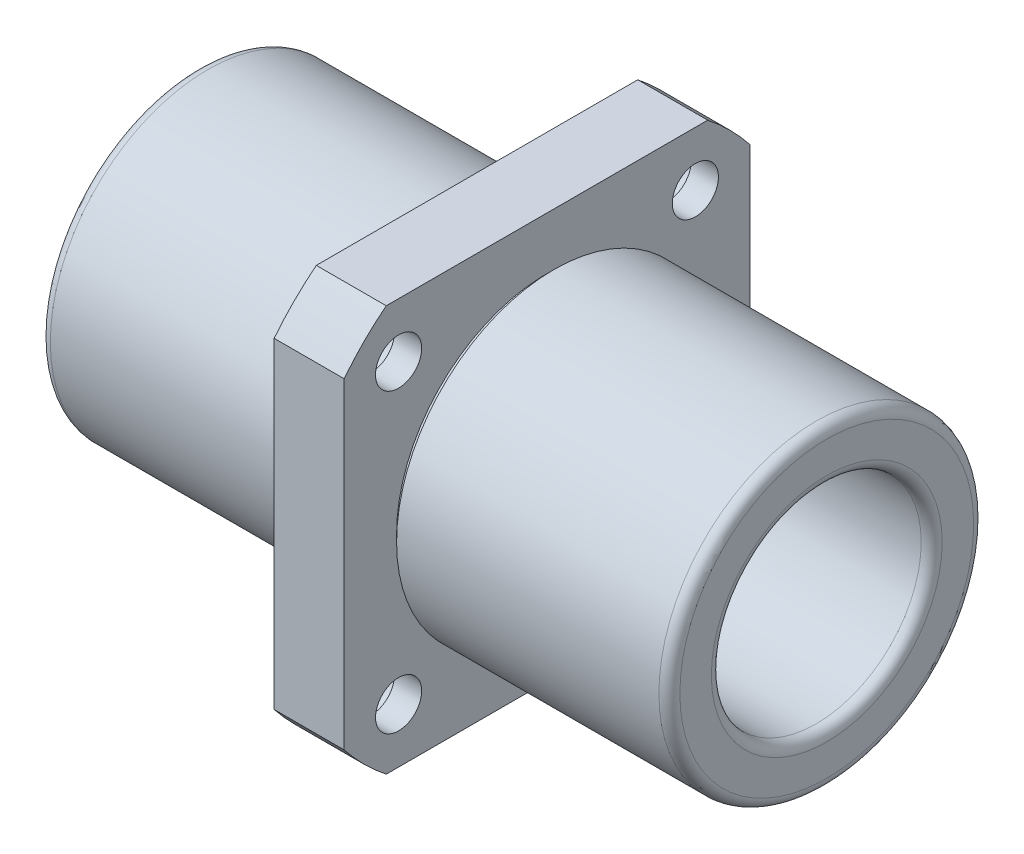
SolidWorks part; units mm, degrees
material "Q235-AF"
ref_plane "Front Plane" through (0, 0, 0) normal (0, 0, 1) x (1, 0, 0)
ref_plane "Top Plane" through (0, 0, 0) normal (0, 1, 0) x (1, 0, 0)
ref_plane "Right Plane" through (0, 0, 0) normal (1, 0, 0) x (0, 0, -1)
sketch "Sketch1" plane through (0, 0, 0) normal (0, 0, 1) x (1, 0, 0)
  line L0 (0, 37) -> (0, 21.5)
  line L1 (0, 15) -> (50, 15)
  line L2 (50, 15) -> (50, 22.5)
  line L3 (50, 22.5) -> (11, 22.5)
  line L4 (11, 22.5) -> (11, 21.5)
  line L5 (11, 21.5) -> (10, 21.5)
  line L6 (10, 21.5) -> (10, 37)
  line L7 (10, 37) -> (0, 37)
  line L8 (64, 0) -> (0, 0) construction
  line L9 (0, 21.5) -> (-1, 21.5)
  line L10 (-1, 21.5) -> (-1, 22.5)
  line L11 (-1, 22.5) -> (-40, 22.5)
  line L12 (-40, 22.5) -> (-40, 15)
  line L13 (-40, 15) -> (0, 15)
  dimension "D4" = 40
  dimension "D1" = 90
  dimension "D2" = 10
  dimension "D3" = 74
  dimension "D5" = 40
  dimension "D6" = 45
  dimension "D7" = 30
  dimension "D8" = 1
  dimension "D9" = 1
revolve "Revolve1" add sketch "Sketch1" angle 360 about L8
sketch "Sketch2" plane through (0, 0, 0) normal (1, 0, 0) x (0, 0, -1)
  line L1 (29, -29) -> (-29, -29)
  line L2 (29, -29) -> (29, 29)
  line L3 (29, 29) -> (-29, 29)
  line L4 (-29, -29) -> (-29, 29)
  line L5 (29, -29) -> (-29, 29) construction
  line L6 (29, 29) -> (-29, -29) construction
  point P0 (0, 0)
  dimension "D1" = 58
extrude "Cut-Extrude1" cut sketch "Sketch2" along normal blind 10 flip side to cut
sketch "Sketch3" plane through (0, 0, 0) normal (-1, 0, 0) x (0, 0, 1)
  line L0 (0, 0) -> (-21.2132, 21.2132) construction
  line L1 (-21.2132, 21.2132) -> (-26.163, 26.163) construction
  circle A0 centre (-21.2132, 21.2132) radius 5.5
  arc A1 (-22.9783, 29) -> (-29, 22.9783) centre (0, 0) ccw construction
  dimension "D2" = 11
  dimension "D1" = 30
extrude "Cut-Extrude2" cut sketch "Sketch3" against normal blind 6.1
sketch "Sketch4" plane through (6.1, 0, 0) normal (-1, 0, 0) x (0, 0, 1)
  circle A0 centre (-21.2132, 21.2132) radius 3.3
  dimension "D1" = 6.6
extrude "Cut-Extrude3" cut sketch "Sketch4" against normal up to next
pattern_circular "CirPattern1" count 4 over 360 about axis through (0, 0, 0) along (1, 0, 0) of "Cut-Extrude3", "Cut-Extrude2"
fillet "Fillet1" radius 1.5 4 edges at (-40, 0, 15) (50, 0, 15) (50, 0, 22.5) (-40, 0, 22.5)
